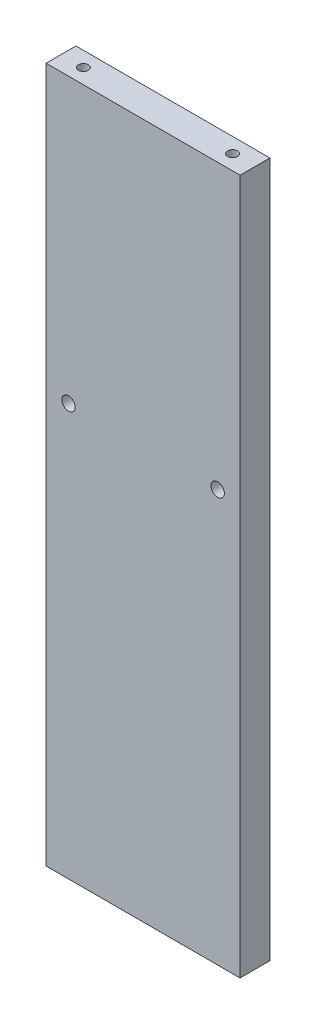
from build123d import *

# Parameters (mm, degrees)
SKETCH_1_W                  = 65
SKETCH_1_H                  = 10
EXTRUDE_1_DEPTH             = 116.5
HOLE_WIZARD_M4_1_AT_2_COUNT = 2
HOLE_WIZARD_M4_1_AT_2_PITCH = 50
HOLE_WIZARD_M4_1_2_D        = 4.5


with BuildPart() as part:
    # 草图1 → 凸台-拉伸1 (new, symmetric)
    with BuildSketch(Plane(origin=(0, 0, 0), x_dir=(1, 0, 0), z_dir=(0, 1, 0))):
        Rectangle(SKETCH_1_W, SKETCH_1_H)
    extrude(amount=EXTRUDE_1_DEPTH, both=True)

    # 草图3 → Hole Wizard M4 _1 (revolve, cut)
    with BuildSketch(Plane(origin=(25, 116.5, 0), x_dir=(0, 0, 1), z_dir=(1, 0, 0))):
        Polygon((0, 0), (0, 11.091420021), (1.65, 10.1), (1.65, 0), align=None)
    hole_wizard_m4_1 = revolve(axis=Axis((25, 122.85, 0), (0, -1, 0)), mode=Mode.SUBTRACT)

    # Hole Wizard M4 _1 at 2: Hole Wizard M4 _1 ×2
    with Locations(*[(-i * HOLE_WIZARD_M4_1_AT_2_PITCH, 0, 0) for i in range(1, HOLE_WIZARD_M4_1_AT_2_COUNT)]):
        add(hole_wizard_m4_1, mode=Mode.SUBTRACT)

    # 镜向1: Hole Wizard M4 _1 across plane
    add(hole_wizard_m4_1.mirror(Plane.ZX), mode=Mode.SUBTRACT)

    # 镜向1 copy 1 sketch → 镜向1 copy 1 (revolve, cut)
    with BuildSketch(Plane(origin=(-25, -116.5, 0), x_dir=(0, 0, 1), z_dir=(1, 0, 0))):
        Polygon((0, 0), (0, -11.091420021), (1.65, -10.1), (1.65, 0), align=None)
    revolve(axis=Axis((-25, -122.85, 0), (0, -1, 0)), mode=Mode.SUBTRACT)

    # Hole Wizard M4 _1 2 (through all)
    with Locations(Plane(origin=(0, 0, -5), x_dir=(-1, 0, 0), z_dir=(0, 0, -1))):
        with Locations((25, 21.5), (-25, 21.5)):
            Hole(HOLE_WIZARD_M4_1_2_D / 2)


solid = part.part
